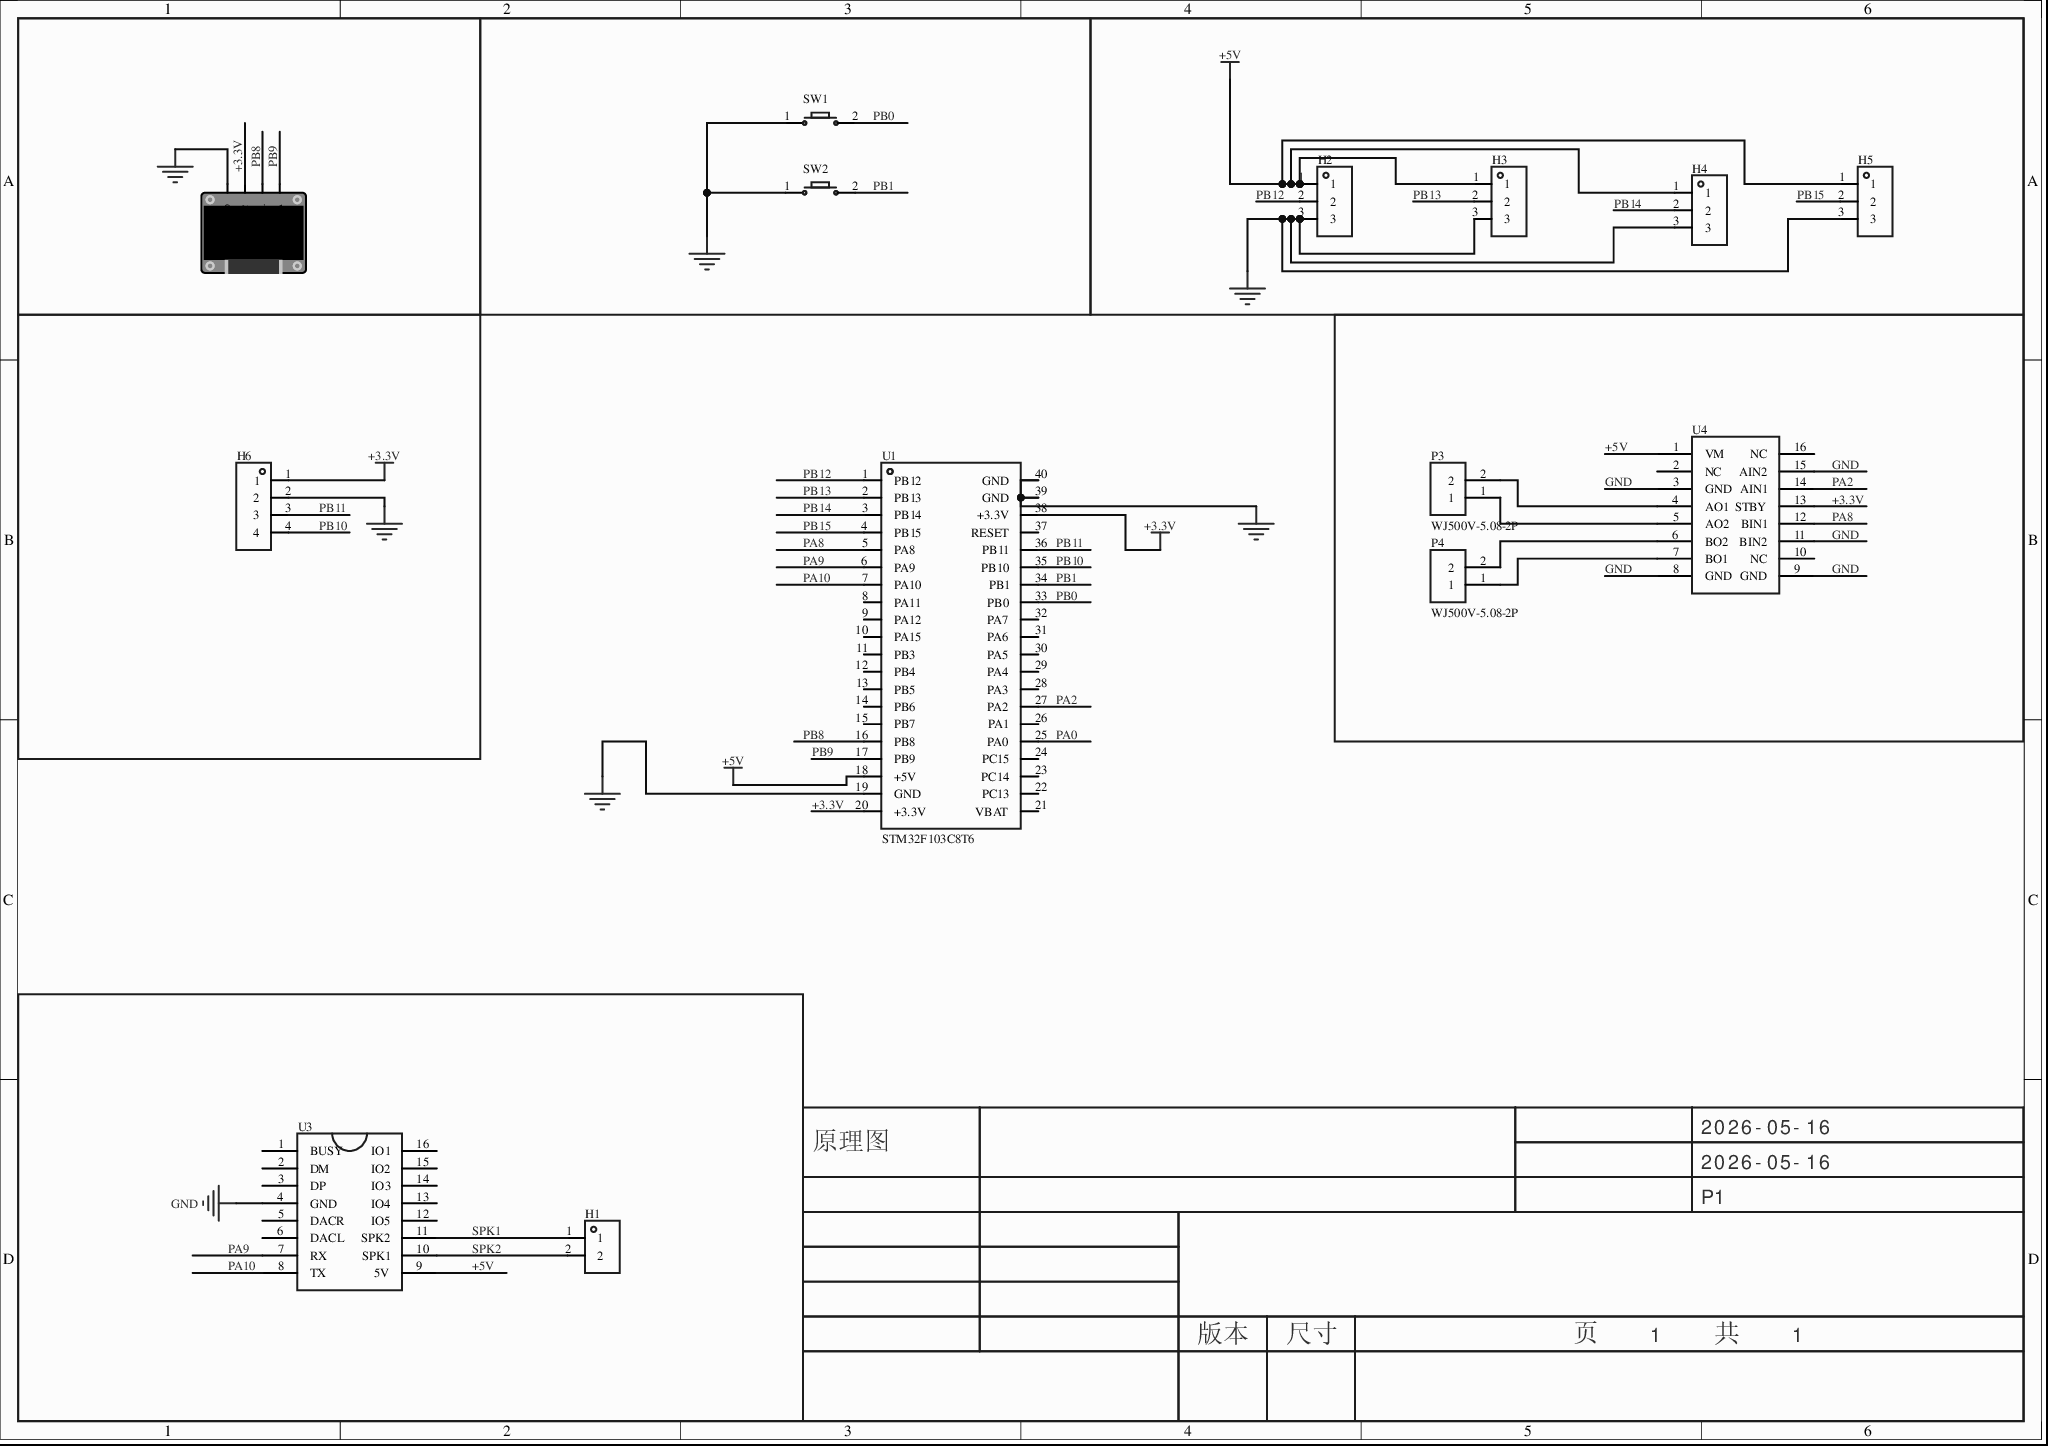
[diagram p0: MISC49887-3.schdoc]
# Altium project MISC49887-2.PrjPcb
1 sheet, 14 parts. Net scope: global (net labels, ports and power ports of the same name join across sheets).
Board file: MISC49887.pcbdoc

## Sheet MISC49887-3.schdoc
size 297 x 209 mm; Version: V1.0; @Project Name: MISC49887; @Page Count: 1; @Update Date: 2026-05-16; @Create Date: 2026-05-16; @Schematic Name: MISC49887; @Page No: 1; @Create Time: 16:23:09; @Update Time: 13:26:11; @Board Name: MISC49887

### Parts
H1  HX PH254-01-02-Z-L11.5 male header connector  [HDR-TH_2P-P2.54-V-M]  (value not drawn)
H2  (no value)  [HDR-TH_3P-P2.54-V-F]
H3  (no value)  [HDR-TH_3P-P2.54-V-F]
H4  (no value)  [HDR-TH_3P-P2.54-V-F]
H5  (no value)  [HDR-TH_3P-P2.54-V-F]
H6  (no value)  [HDR-TH_4P-P2.54-V-F]
OLED1  (no value)  [0.96OLED_4P]
P3  WJ500V-5.08-2P  [CONN-TH_2P-P5.00_WJ500V-5.08-2P]
P4  WJ500V-5.08-2P  [CONN-TH_2P-P5.00_WJ500V-5.08-2P]
SW1  (no value)  [Key_SMD_3x4x2]
SW2  (no value)  [Key_SMD_3x4x2]
U1  STM32F103C8T6  [CONN-TH_L53.3-W22.9_STM32F103C8T6-CARD]
U3  (no value)  [MY2490-16P]
U4  (no value)  [DRV8833]

### Nets
+3.3V: H6.1 OLED1.2(VCC) U1.20(+3.3V) U1.38(+3.3V) U4.13(STBY)
+5V: H2.1 H3.1 H4.1 H5.1 U1.18(+5V) U3.9(5V) U4.1(VM)
GND: H2.3 H3.3 H4.3 H5.3 H6.2 OLED1.1(GND) SW1.1 SW2.1 U1.19(GND) U1.39(GND) U1.40(GND) U3.4(GND) U4.3(GND) U4.8(GND) U4.9(GND) U4.11(BIN2) U4.15(AIN2)
PA0: U1.25(PA0)
PA2: U1.27(PA2) U4.14(AIN1)
PA8: U1.5(PA8) U4.12(BIN1)
PA9: U1.6(PA9) U3.7(RX)
PA10: U1.7(PA10) U3.8(TX)
PB0: SW1.2 U1.33(PB0)
PB1: SW2.2 U1.34(PB1)
PB8: OLED1.3(SCL) U1.16(PB8)
PB9: OLED1.4(SDA) U1.17(PB9)
PB10: H6.4 U1.35(PB10)
PB11: H6.3 U1.36(PB11)
PB12: H2.2 U1.1(PB12)
PB13: H3.2 U1.2(PB13)
PB14: H4.2 U1.3(PB14)
PB15: H5.2 U1.4(PB15)
SPK1: H1.1 U3.11(SPK2)
SPK2: H1.2 U3.10(SPK1)
NetP3_1: P3.1 U4.5(AO2)
NetP3_2: P3.2 U4.4(AO1)
NetP4_1: P4.1 U4.7(BO1)
NetP4_2: P4.2 U4.6(BO2)

Not connected (* = marked no-connect by the designer): U1 8(PA11) 9(PA12)* 10(PA15)* 11(PB3)* 12(PB4)* 13(PB5)* 14(PB6)* 15(PB7)* 21(VBAT)* 22(PC13)* 23(PC14)* 24(PC15)* 26(PA1)* 28(PA3)* 29(PA4)* 30(PA5)* 31(PA6)* 32(PA7)* 37(RESET); U3 1(BUSY) 2(DM) 3(DP) 5(DACR) 6(DACL) 12(IO5) 13(IO4) 14(IO3) 15(IO2) 16(IO1); U4 2(NC) 10(NC) 16(NC)

### Notes on the sheet
- 2026-05-16
- 原理图
- P1
- 版本
- 尺寸
- 页    1    共    1

### Library data of the parts
H1 = HX PH254-01-02-Z-L11.5 male header connector: 插针结构:1x2P;间距:2.54mm;圆针/方针:方针;安装方式:直插;排数:单排;总PIN位数:2P;额定电流:3A;额定电压:1kV;配合针长度:6mm;塑高:2.5mm;端接针长度:3mm;触头材质:黄铜;触头镀层:金;工作温度:-40℃~+105℃;; Manufacturer: hanxia(韩下); 3D Model: e35305ec3aa84b66b849f914b715e73f0819f05c4eef4c71ace90d822a990e87; 3D Model Transform: 200,100,0,0,0,0,0,0,-118.11; Pin Structure: 1x2P; Pitch: 2.54mm; Circluar Pins/Square Pins: 方针; Current Rating: 3A; Voltage Rating (Max): 1kV; AddInBom: yes; ModelName: HDR2.54-M-LI-1X2P; Symbol: HX PH254-01-02-Z-L11.5 MALE HEADER CONNECTOR; Device: HX PH254-01-02-Z-L11.5 male header connector; LCSC Part Name: 1x2P 间距:2.54mm 方针 直插; Supplier Part: C52016390; Manufacturer Part: HX PH254-01-02-Z-L11.5 male header connector; Supplier Footprint: 插件,P=2.54mm; JLCPCB Part Class: Extended Part; Datasheet: https://item.szlcsc.com/datasheet/HX%2520PH254-01-02-Z-L11.5%2520male%2520header%2520connector/54760435.html; Supplier: LCSC; Mounting Type: 直插; Number of Rows: 单排; Number of Pins: 2P; Length of Mating Pin: 6mm; Insulation Height: 2.5mm; Length of End Connection Pin: 3mm; Contact Material: 黄铜; Contact Plating: 金; Operating Temperature: -40℃~+105℃; ConvertToPcb: yes; FootprintName: HDR-TH_2P-P2.54-V-M
H2-H5 = HDR-F_2.54_1x3P: Symbol: PM254V-11-03-H85; ConvertToPcb: yes; ModelId: f3b3cc5aae9641bf9e56fc160cef875b0819f05c4eef4c71ace90d822a990e87; ModelName: HDR2.54-F-LI-1X3P; ModelTransform: 299.9994,100,0,0,0,0,0,0,-118.11; Device: HDR-F_2.54_1x3P; AddInBom: yes; SupplierPart: C541850; Supplier Footprint: 插件; FootprintName: HDR-TH_3P-P2.54-V-F
H6 = HDR-F_2.54_1x4P: Symbol: 2.54-1*4P母; ConvertToPcb: yes; ModelId: d187812051054f85879fcaa51a310d8e0819f05c4eef4c71ace90d822a990e87; ModelTransform: 419.6842,98.464,0,0,0,0,0,0,-118.11; Device: HDR-F_2.54_1x4P; AddInBom: yes; SupplierPart: C2718488; Supplier Footprint: 插件; FootprintName: HDR-TH_4P-P2.54-V-F; ModelName: HDR-TH_4P-P2.54-V-F
OLED1 = 0.96OLED模块_4P: ConvertToPcb: yes; ModelId: 79c000fdb68d45a296c2e9bedf4f9055; ModelTransform: 1393.69792,1318.895,0,0,0,0,0,-560.079,-137.795; Device: 0.96OLED模块_4P; Symbol: 0.96OLED模块_4P; AddInBom: yes; FootprintName: 0.96OLED_4P; Supplier Footprint: 插件; ModelName: 0.96OLED_4P
P3 P4 = WJ500V-5.08-2P: 结构:1x2P;间距:5.08mm;颜色:绿色;安装方式:直插;额定电流:18A;额定电压:250V;排数:1;线规 - AWG:14~30;线规 - 平方毫米:2.5;每排PIN数:2;触头材质:-;触头镀层:-;工作温度范围:-40℃~+105℃;焊接温度(最大值):-;; Manufacturer: KANGNEX(康奈克斯电气); Symbol: WJ500V-5.08-2P-14-00A; 3D Model: 0f4a503c8d3b4ae19ed61267f5e9a1d70819f05c4eef4c71ace90d822a990e87; 3D Model Transform: 423.621,393.7,0,0,0,0,-11.811,19.685,-137.795; Structure: 1x2P; Pitch: 5.08mm; Current Rating (Max): 18A; Voltage Rating (Max): 250V; Wire Gauge - AWG: 14~30; Wire Gauge - mm2: 2.5; Number of PINs Per Row: 2; Screw Specification: M2.5; AddInBom: yes; Device: WJ500V-5.08-2P; LCSC Part Name: 1x2P 5.08mm 直插 排数:1 每排P数:2; Supplier Part: C8465; Manufacturer Part: WJ500V-5.08-2P; Supplier Footprint: 插件,P=5.08mm; JLCPCB Part Class: Extended Part; Datasheet: https://atta.szlcsc.com/upload/public/pdf/source/20191225/C8465_02D34CE5B5B4A53DF5891601D97FA9F4.pdf; Supplier: LCSC; Color: 绿色; Mounting Style: 直插; Number of Pins: 2P; Number of Rows: 1; Contact Material: -; Contact Plating: -; Operating Temperature Range: -40℃~+105℃; Soldering Temperature(Max): -; ConvertToPcb: yes; FootprintName: CONN-TH_2P-P5.00_WJ500V-5.08-2P; ModelName: CONN-TH_2P-P5.00_WJ500V-5.08-2P
SW1 = Key_SMD_3x4x2: Symbol: 轻触按键x2; 3D Model: 63599cce708d48afbce1b0db003544770819f05c4eef4c71ace90d822a990e87; 3D Model Transform: 196.85,114.17,79.13,0,0,0,0,0,0; ConvertToPcb: yes; ModelName: SW-SMD_L4.0-W2.9-H2-LS5.0; Device: Key_SMD_3x4x2; Supplier Footprint: SMD; AddInBom: yes; FootprintName: Key_SMD_3x4x2
SW2 = Key_SMD_3x4x2: Symbol: 轻触按键x2; ConvertToPcb: yes; ModelId: 63599cce708d48afbce1b0db003544770819f05c4eef4c71ace90d822a990e87; ModelName: SW-SMD_L4.0-W2.9-H2-LS5.0; ModelTransform: 196.85,114.17,79.13,0,0,0,0,0,0; Device: Key_SMD_3x4x2; AddInBom: yes; Supplier Footprint: SMD; FootprintName: Key_SMD_3x4x2
U1 = LCKFB-DKX-STM32F103C8T6: Manufacturer: 立创开发板; AddInBom: yes; ModelId: 12c257eccf3b4e5baa9346e6693d8ea40819f05c4eef4c71ace90d822a990e87; Symbol: LCKFB-DKX-STM32F103C8T6; Manufacturer Part: STM32F103C8T6; Device: LCKFB-DKX-STM32F103C8T6; LCSC Part Name: 立创·地阔星-STM32F103C8T6开发板; SupplierPart: C22396880; Supplier Footprint: -; JLCPCB Part Class: 扩展库; Datasheet: https://atta.szlcsc.com/upload/public/pdf/source/20240801/7EEF69F7480DF7C6DA98696664D658D4.pdf; Supplier: LCSC; ConvertToPcb: yes; FootprintName: CONN-TH_L53.3-W22.9_STM32F103C8T6-CARD; ModelName: CONN-TH_L53.3-W22.9_STM32F103C8T6-CARD
U3 = MY2490-16PMP3语言播放: AddInBom: yes; ModelTransform: 0, 0, 0, 0, 0, 0, 0, 0, 0; Symbol: MY2490-16PMP3语言播放; Device: MY2490-16PMP3语言播放; ConvertToPcb: yes; FootprintName: MY2490-16P
U4 = DRV8833: AddInBom: yes; Symbol: DRV8833; Device: DRV8833; ConvertToPcb: yes; FootprintName: DRV8833